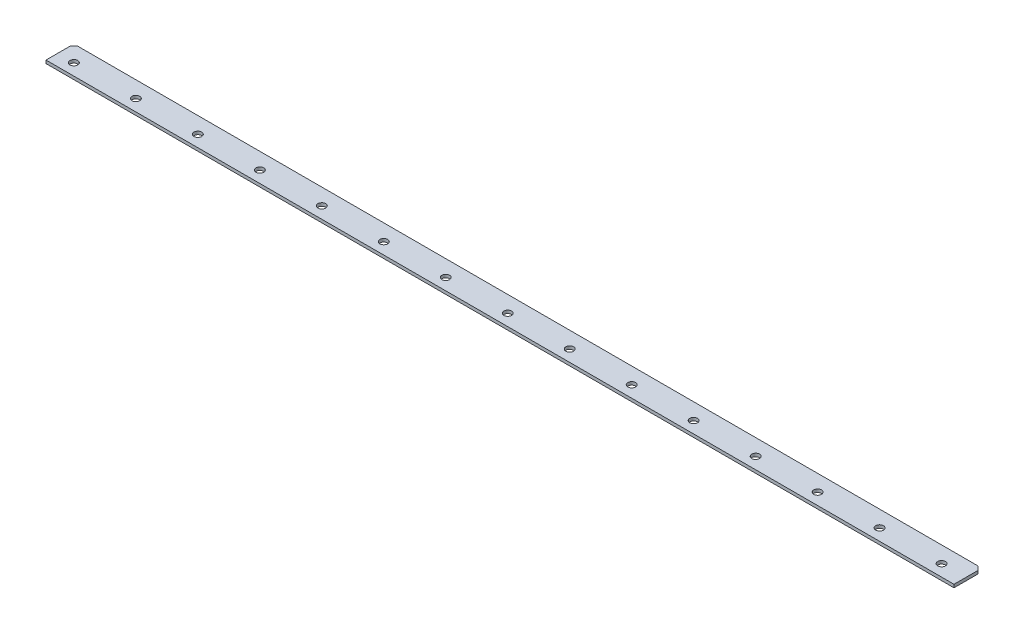
SolidWorks part; units mm, degrees
material "Q235"
ref_plane "前视基准面" through (0, 0, 0) normal (0, 0, 1) x (1, 0, 0)
ref_plane "上视基准面" through (0, 0, 0) normal (0, 1, 0) x (1, 0, 0)
ref_plane "右视基准面" through (0, 0, 0) normal (1, 0, 0) x (0, 0, -1)
sketch "草图1" plane through (0, 0, 0) normal (0, 1, 0) x (1, 0, 0)
  line L0 (-2.2, 0) -> (2.2, 0) construction
  line L1 (-1172, 0) -> (0, 0)
  line L2 (-1172, 0) -> (-1172, -36)
  line L3 (-1172, -36) -> (0, -36)
  line L4 (0, 0) -> (0, -36)
  line L5 (0, -2.2) -> (0, 2.2) construction
  dimension "D1" = 36
  dimension "D2" = 1172
extrude "凸台-拉伸1" add sketch "草图1" along normal blind 4
chamfer "倒角1" distance 5 angle 45 2 edges at (0, 2, 0) (-1172, 2, 0)
hole_wizard "Ø10.0 (10) 直径孔1" positions "草图4" profile "草图3" hole size "Ø10.0" standard "GB" end condition through all
sketch "草图4" plane through (0, 4, 0) normal (0, 1, 0) x (-1, 0, 0)
  line L0 (1172, 36) -> (0, 36) construction
  line L2 (1172, 5) -> (1172, 36) construction
  point P0 (1151, 21)
  dimension "D1" = 15
  dimension "D2" = 21
sketch "草图3" plane through (-1151, 4, 21) normal (1, 0, 0) x (0, 0, 1)
  line L0 (0, 0) -> (0, 4)
  line L1 (0, 4) -> (5, 4)
  line L2 (5, 4) -> (5, 0)
  line L5 (5, 0) -> (0, 0)
  line L11 (0, -6.35) -> (0, 107.95) construction
  dimension "通孔孔直径" = 10
  dimension "通孔孔深度" = 4
pattern_linear "阵列(线性)1" count 15 spacing 80 along (1, 0, 0) of "Ø10.0 (10) 直径孔1"
